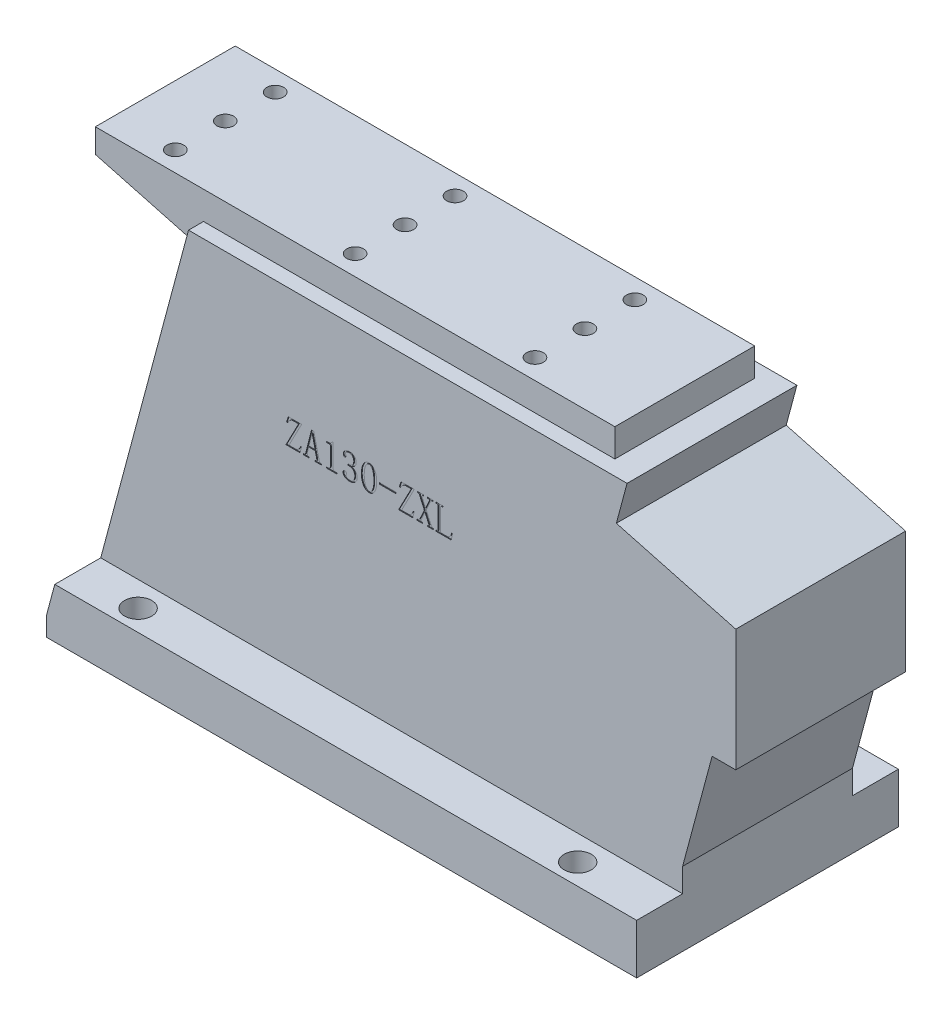
from build123d import *

# Parameters (mm, degrees)
BOSS_EXTRUDE1_DEPTH   = 21.25
SKETCH2_W             = 130
SKETCH2_H             = 3.75
CUT_EXTRUDE1_DEPTH    = 7
CUT_EXTRUDE2_DEPTH    = 3.75
CUT_EXTRUDE3_DEPTH    = 3.75
BOSS_EXTRUDE2_DEPTH   = 32.75
M8_TAPPED_HOLE1_D     = 6.8
M5_TAPPED_HOLE1_D     = 4.2
M5_TAPPED_HOLE1_DEPTH = 12.4
M5_TAPPED_HOLE1_TIP   = 1.2618073
SKETCH10_W            = 4.088356164
SKETCH10_H            = 0.347945206
CUT_EXTRUDE4_DEPTH    = 0.2
SKETCH11_R            = 3
OUTLET_POSITION_DEPTH = 12


with BuildPart() as part:
    # Sketch1 → Boss-Extrude1 (new, symmetric)
    with BuildSketch(Plane.XY):
        Polygon((0, 0), (-130, 0), (-130, -6), (-104.5, -12.832704407), (-127, -96.803847577), (-127, -101.5), (20.7, -101.5), (20.7, -83.052861599), (28.082767015, -55.5), (34, -55.5), (34, -25), (4.124054476, -16.994764524), (6.802143559, -7), (0, -7), align=None)
    extrude(amount=BOSS_EXTRUDE1_DEPTH, both=True)

    # Sketch2 → Cut-Extrude1 (cut)
    with BuildSketch(Plane(origin=(0, 0, 0), x_dir=(1, 0, 0), z_dir=(0, 1, 0))):
        with Locations((-65, 19.375)):
            Rectangle(SKETCH2_W, SKETCH2_H)
        with Locations((-65, -19.375)):
            Rectangle(SKETCH2_W, SKETCH2_H)
    extrude(amount=-CUT_EXTRUDE1_DEPTH, mode=Mode.SUBTRACT)

    # Sketch3 → Cut-Extrude2 (cut)
    with BuildSketch(Plane.XY.offset(21.25)):
        Polygon((-104.5, -12.832704407), (-102.937131564, -7), (-126.267949192, -7), align=None)
    extrude(amount=-CUT_EXTRUDE2_DEPTH, mode=Mode.SUBTRACT)

    # Sketch4 → Cut-Extrude3 (cut)
    with BuildSketch(Plane(origin=(0, 0, -21.25), x_dir=(-1, 0, 0), z_dir=(0, 0, -1))):
        Polygon((102.937131564, -7), (104.5, -12.832704407), (126.267949192, -7), align=None)
    extrude(amount=-CUT_EXTRUDE3_DEPTH, mode=Mode.SUBTRACT)

    # Sketch5 → Boss-Extrude2 (add, symmetric)
    with BuildSketch(Plane.XY):
        Polygon((20.7, -101.5), (20.7, -89), (-124.908965344, -89), (-127, -96.803847577), (-127, -101.5), align=None)
    extrude(amount=BOSS_EXTRUDE2_DEPTH, both=True)

    # M8 Tapped Hole1 (through all)
    with Locations(Plane(origin=(0, -101.5, 0), x_dir=(-1, 0, 0), z_dir=(0, -1, 0))):
        with Locations((-0.7, -27.5), (109.3, -27.5), (-0.7, 27.5), (109.3, 27.5)):
            Hole(M8_TAPPED_HOLE1_D / 2)

    # M5 Tapped Hole1
    with Locations(Plane(origin=(0, 0, 0), x_dir=(1, 0, 0), z_dir=(0, 1, 0))):
        with Locations((-25, 0), (-115, 12.5), (-115, -12.5), (-115, 0), (-70, 12.5), (-70, -12.5), (-70, 0), (-25, 12.5), (-25, -12.5)):
            Hole(M5_TAPPED_HOLE1_D / 2, depth=M5_TAPPED_HOLE1_DEPTH)
            with Locations((0, 0, -(M5_TAPPED_HOLE1_DEPTH + M5_TAPPED_HOLE1_TIP / 2))):  # 118° drill point
                Cone(0, M5_TAPPED_HOLE1_D / 2, M5_TAPPED_HOLE1_TIP, mode=Mode.SUBTRACT)

    # Sketch10 → Cut-Extrude4 (cut)
    # profile 1 of 9: a face of its own
    with BuildSketch(Plane.XY.offset(21.25)):
        with BuildLine():
            add(Edge.make_bspline(
                [(-76.242874665, -41.028711733), (-76.203886828, -41.027431457), (-76.127040008, -41.024907974), (-76.013494906, -41.011969414), (-75.904757802, -40.986452399), (-75.798985146, -40.954804143), (-75.698746914, -40.910149848), (-75.600937291, -40.859034731), (-75.509116676, -40.795612853), (-75.419480888, -40.724507175), (-75.334714639, -40.643281232), (-75.253475154, -40.552312423), (-75.176950666, -40.451930765), (-75.10230024, -40.343014665), (-75.03582371, -40.222632516), (-74.969440865, -40.094612706), (-74.908945483, -39.95631791), (-74.872425189, -39.859995456), (-74.853812165, -39.810903514)],
                knots=[0, 0, 0, 0, 0.944510353, 1.861673376, 2.761280467, 3.64611623, 4.530611868, 5.414086345, 6.314763123, 7.227980775, 8.182441956, 9.153653734, 10.17841272, 11.237309815, 12.347695367, 13.505623519, 14.728709846, 16, 16, 16, 16], degree=3))
            Line((-74.853812165, -39.810903514), (-74.63498725, -39.810903514))
            Line((-74.63498725, -39.810903514), (-75.037298894, -41.289670637))
            Line((-75.037298894, -41.289670637), (-78.549370812, -41.289670637))
            Line((-78.549370812, -41.289670637), (-75.368934168, -35.200629541))
            Line((-75.368934168, -35.200629541), (-76.637031343, -35.200629541))
            add(Edge.make_bspline(
                [(-76.637031343, -35.200629541), (-76.713929015, -35.20386524), (-76.86554004, -35.210244727), (-77.0867771, -35.266142831), (-77.296788501, -35.354772843), (-77.494614616, -35.481230446), (-77.680673118, -35.64201888), (-77.853401182, -35.839278631), (-78.016181535, -36.070275987), (-78.109407187, -36.242043857), (-78.157932456, -36.331451459)],
                knots=[0, 0, 0, 0, 0.92088507, 1.815611915, 2.718761103, 3.64423436, 4.618919569, 5.657996246, 6.78095397, 8, 8, 8, 8], degree=3))
            Line((-78.157932456, -36.331451459), (-78.375398209, -36.244465158))
            Line((-78.375398209, -36.244465158), (-77.939107541, -34.939670637))
            Line((-77.939107541, -34.939670637), (-74.63498725, -34.939670637))
            Line((-74.63498725, -34.939670637), (-77.815423894, -41.028711733))
            Line((-77.815423894, -41.028711733), (-76.242874665, -41.028711733))
        make_face()
    # profile 2 of 9: a face of its own
    with BuildSketch(Plane.XY.offset(21.25)):
        with BuildLine():
            Line((-71.216697439, -38.9410405), (-72.865359682, -38.9410405))
            Line((-72.865359682, -38.9410405), (-73.195635795, -40.298842298))
            add(Edge.make_bspline(
                [(-73.195635795, -40.298842298), (-73.201385906, -40.327331199), (-73.212207931, -40.380948874), (-73.222817521, -40.457693122), (-73.230212975, -40.525684008), (-73.231658112, -40.568393726), (-73.232333141, -40.588343582)],
                knots=[0, 0, 0, 0, 1.193188097, 2.245645547, 3.180534975, 4, 4, 4, 4], degree=3))
            add(Edge.make_bspline(
                [(-73.232333141, -40.588343582), (-73.229172539, -40.637388853), (-73.222745637, -40.737119608), (-73.193404116, -40.860269091), (-73.140700756, -40.950837825), (-73.069099444, -40.998644876), (-72.97445228, -41.024203716), (-72.904047344, -41.027113049), (-72.865359682, -41.028711733)],
                knots=[0, 0, 0, 0, 1.327183477, 2.698751724, 3.381033576, 4.100799874, 4.956385495, 6, 6, 6, 6], degree=3))
            Line((-72.865359682, -41.028711733), (-72.755267644, -41.028711733))
            Line((-72.755267644, -41.028711733), (-72.755267644, -41.289670637))
            Line((-72.755267644, -41.289670637), (-74.113069442, -41.289670637))
            Line((-74.113069442, -41.289670637), (-74.113069442, -41.028711733))
            Line((-74.113069442, -41.028711733), (-74.002977404, -41.028711733))
            add(Edge.make_bspline(
                [(-74.002977404, -41.028711733), (-73.979277578, -41.027869149), (-73.932540679, -41.026207544), (-73.865457949, -41.006905979), (-73.80171868, -40.980398661), (-73.743506339, -40.940084995), (-73.69235851, -40.885762933), (-73.649466648, -40.816358215), (-73.619058841, -40.729997868), (-73.606186651, -40.666913718), (-73.5993066, -40.633195894)],
                knots=[0, 0, 0, 0, 0.909603974, 1.793771294, 2.668600383, 3.558767937, 4.496366253, 5.522416659, 6.675757406, 8, 8, 8, 8], degree=3))
            Line((-73.5993066, -40.633195894), (-72.169469271, -34.939670637))
            Line((-72.169469271, -34.939670637), (-71.620368243, -34.852684336))
            Line((-71.620368243, -34.852684336), (-70.22722826, -40.626400089))
            add(Edge.make_bspline(
                [(-70.22722826, -40.626400089), (-70.214798708, -40.660671284), (-70.191446746, -40.725058124), (-70.147952049, -40.811446769), (-70.100303286, -40.882599979), (-70.047026521, -40.938135249), (-69.987813356, -40.978759842), (-69.924729189, -41.007250277), (-69.857252558, -41.026105198), (-69.810545038, -41.027834713), (-69.78686011, -41.028711733)],
                knots=[0, 0, 0, 0, 1.359311801, 2.55380043, 3.599420041, 4.543802956, 5.406592952, 6.26139706, 7.118371362, 8, 8, 8, 8], degree=3))
            Line((-69.78686011, -41.028711733), (-69.676768072, -41.028711733))
            Line((-69.676768072, -41.028711733), (-69.676768072, -41.289670637))
            Line((-69.676768072, -41.289670637), (-71.254753945, -41.289670637))
            Line((-71.254753945, -41.289670637), (-71.254753945, -41.028711733))
            Line((-71.254753945, -41.028711733), (-71.107964562, -41.028711733))
            add(Edge.make_bspline(
                [(-71.107964562, -41.028711733), (-71.074722312, -41.028173841), (-71.015782969, -41.027220145), (-70.938845974, -41.009815927), (-70.880539429, -40.983149607), (-70.84058845, -40.926410966), (-70.822653035, -40.854167587), (-70.816982114, -40.797688263), (-70.814385795, -40.771830312)],
                knots=[0, 0, 0, 0, 1.306477298, 2.316417055, 3.107965527, 3.758448528, 4.973749602, 6, 6, 6, 6], degree=3))
            add(Edge.make_bspline(
                [(-70.814385795, -40.771830312), (-70.815629301, -40.725782798), (-70.817957288, -40.639576536), (-70.840555758, -40.556409946), (-70.851083141, -40.517667213)],
                knots=[0, 0, 0, 0, 1.068310181, 2, 2, 2, 2], degree=3))
            Line((-70.851083141, -40.517667213), (-71.216697439, -38.9410405))
        make_face()
        Polygon((-71.985982541, -35.563525517), (-72.022679887, -35.563525517), (-72.79196499, -38.680081596), (-71.253394784, -38.680081596), align=None, mode=Mode.SUBTRACT)
    # profile 3 of 9: a face of its own
    with BuildSketch(Plane.XY.offset(21.25)):
        with BuildLine():
            Line((-66.806220127, -34.852684336), (-66.806220127, -40.440195038))
            add(Edge.make_bspline(
                [(-66.806220127, -40.440195038), (-66.80467875, -40.486687653), (-66.801754974, -40.57487759), (-66.765206281, -40.697367598), (-66.707173198, -40.801979197), (-66.624651324, -40.88647853), (-66.521171511, -40.95075514), (-66.399845762, -40.99681991), (-66.260091344, -41.02370043), (-66.161195339, -41.026979912), (-66.108970555, -41.028711733)],
                knots=[0, 0, 0, 0, 1.071056132, 2.031642504, 2.922379843, 3.810776537, 4.728479874, 5.716066906, 6.793905654, 8, 8, 8, 8], degree=3))
            Line((-66.108970555, -41.028711733), (-65.741997096, -41.028711733))
            Line((-65.741997096, -41.028711733), (-65.741997096, -41.289670637))
            Line((-65.741997096, -41.289670637), (-68.442649921, -41.289670637))
            Line((-68.442649921, -41.289670637), (-68.442649921, -41.028711733))
            Line((-68.442649921, -41.028711733), (-68.112373808, -41.028711733))
            add(Edge.make_bspline(
                [(-68.112373808, -41.028711733), (-68.055160572, -41.02707448), (-67.948596144, -41.024024958), (-67.801293568, -40.997405203), (-67.677912998, -40.953587743), (-67.579028914, -40.8883489), (-67.504418159, -40.80282752), (-67.450235877, -40.700325183), (-67.421300953, -40.578541929), (-67.417258166, -40.492439055), (-67.415124236, -40.446990843)],
                knots=[0, 0, 0, 0, 1.316051353, 2.45125549, 3.431393499, 4.310694105, 5.145582167, 6.017928727, 6.953791053, 8, 8, 8, 8], degree=3))
            Line((-67.415124236, -40.446990843), (-67.415124236, -36.050105141))
            add(Edge.make_bspline(
                [(-67.415124236, -36.050105141), (-67.415945488, -36.02686197), (-67.417534132, -35.981899959), (-67.436165212, -35.918269114), (-67.464891325, -35.860912516), (-67.506211557, -35.81159128), (-67.558943345, -35.77127469), (-67.623554665, -35.742634771), (-67.699146587, -35.72483495), (-67.75344712, -35.723337466), (-67.782097695, -35.72254735)],
                knots=[0, 0, 0, 0, 0.998431823, 1.931384586, 2.83044576, 3.74504897, 4.678001734, 5.664921659, 6.767943239, 8, 8, 8, 8], degree=3))
            Line((-67.782097695, -35.72254735), (-68.442649921, -35.72254735))
            Line((-68.442649921, -35.72254735), (-68.442649921, -35.461588445))
            Line((-68.442649921, -35.461588445), (-68.112373808, -35.461588445))
            add(Edge.make_bspline(
                [(-68.112373808, -35.461588445), (-68.042041194, -35.459948587), (-67.907537058, -35.45681252), (-67.7159154, -35.42814996), (-67.544083534, -35.38151405), (-67.391738478, -35.313706281), (-67.256629308, -35.227899375), (-67.139864476, -35.120764029), (-67.037235987, -34.996458), (-66.985047444, -34.901225686), (-66.958446154, -34.852684336)],
                knots=[0, 0, 0, 0, 1.220065567, 2.333254132, 3.353979704, 4.300888212, 5.216996827, 6.11885441, 7.041151654, 8, 8, 8, 8], degree=3))
            Line((-66.958446154, -34.852684336), (-66.806220127, -34.852684336))
        make_face()
    # profile 4 of 9: a face of its own
    with BuildSketch(Plane.XY.offset(21.25)):
        with BuildLine():
            add(Edge.make_bspline(
                [(-60.717179031, -39.525479713), (-60.718632719, -39.583122003), (-60.721496409, -39.696674284), (-60.747683396, -39.863945469), (-60.785780016, -40.026659684), (-60.84458396, -40.183418132), (-60.915732944, -40.336227421), (-61.00571177, -40.482588724), (-61.110480389, -40.624274897), (-61.230837318, -40.759053152), (-61.363979104, -40.8850466), (-61.514099457, -40.992040255), (-61.674525485, -41.085644865), (-61.848763453, -41.159952901), (-62.034728022, -41.219353865), (-62.234102437, -41.258406897), (-62.4457243, -41.28588111), (-62.591366388, -41.28838422), (-62.666215846, -41.289670637)],
                knots=[0, 0, 0, 0, 0.939588951, 1.85094084, 2.756099325, 3.660865542, 4.576551747, 5.501761, 6.458057624, 7.447364816, 8.446121927, 9.440961631, 10.44742643, 11.470200686, 12.524293599, 13.62578974, 14.779828329, 16, 16, 16, 16], degree=3))
            add(Edge.make_bspline(
                [(-62.666215846, -41.289670637), (-62.720648414, -41.28885503), (-62.827548627, -41.287253257), (-62.98445019, -41.267838117), (-63.13641713, -41.2424934), (-63.281610177, -41.200086677), (-63.422710616, -41.150685482), (-63.55715243, -41.087810708), (-63.685575093, -41.013815991), (-63.806948356, -40.930725812), (-63.91740262, -40.838712828), (-64.015600037, -40.743079357), (-64.097976582, -40.643140114), (-64.165254558, -40.540081082), (-64.219681891, -40.434004815), (-64.255334047, -40.322736055), (-64.280519407, -40.209360298), (-64.282583011, -40.13225689), (-64.283617387, -40.093608993)],
                knots=[0, 0, 0, 0, 1.178422216, 2.31430543, 3.421283865, 4.511956533, 5.586120769, 6.657546332, 7.721528688, 8.794167313, 9.839701404, 10.832154961, 11.759582411, 12.638864268, 13.494774353, 14.332771034, 15.164305512, 16, 16, 16, 16], degree=3))
            add(Edge.make_bspline(
                [(-64.283617387, -40.093608993), (-64.281964891, -40.058028558), (-64.278729816, -39.988373108), (-64.247767013, -39.888342875), (-64.202225676, -39.793835003), (-64.134658042, -39.712443263), (-64.062157498, -39.641286677), (-63.984698109, -39.590677598), (-63.908279812, -39.555015851), (-63.855381914, -39.551603863), (-63.829657627, -39.54994461)],
                knots=[0, 0, 0, 0, 1.101766282, 2.156916416, 3.226505383, 4.338286303, 5.423034469, 6.367313602, 7.206023381, 8, 8, 8, 8], degree=3))
            add(Edge.make_bspline(
                [(-63.829657627, -39.54994461), (-63.794496502, -39.551317894), (-63.727550751, -39.553932586), (-63.63588479, -39.585713227), (-63.559963781, -39.638421443), (-63.50763681, -39.711338831), (-63.467382417, -39.786572696), (-63.436808565, -39.857360708), (-63.417296152, -39.921763456), (-63.414876668, -39.96302044), (-63.413754373, -39.982157795)],
                knots=[0, 0, 0, 0, 1.261452964, 2.401769415, 3.443008139, 4.53625006, 5.594855579, 6.516052044, 7.311659842, 8, 8, 8, 8], degree=3))
            add(Edge.make_bspline(
                [(-63.413754373, -39.982157795), (-63.414350208, -40.010768638), (-63.415492744, -40.065631085), (-63.429231137, -40.143365007), (-63.451349155, -40.212949651), (-63.475497074, -40.252550603), (-63.487149065, -40.271659079)],
                knots=[0, 0, 0, 0, 1.131339522, 2.169389213, 3.1166833, 4, 4, 4, 4], degree=3))
            add(Edge.make_bspline(
                [(-63.487149065, -40.271659079), (-63.498740934, -40.294480658), (-63.520738347, -40.337788234), (-63.541137591, -40.404251701), (-63.558510961, -40.46468712), (-63.55989365, -40.504421644), (-63.560543757, -40.523103856)],
                knots=[0, 0, 0, 0, 1.159795864, 2.200897025, 3.154105307, 4, 4, 4, 4], degree=3))
            add(Edge.make_bspline(
                [(-63.560543757, -40.523103856), (-63.557169653, -40.558716386), (-63.550391972, -40.630252528), (-63.49168159, -40.729179466), (-63.402007862, -40.817158468), (-63.279651686, -40.889131327), (-63.139875823, -40.950482171), (-62.988600468, -40.994873139), (-62.830375755, -41.023294596), (-62.722518295, -41.026883515), (-62.667575007, -41.028711733)],
                knots=[0, 0, 0, 0, 0.760241701, 1.527124279, 2.408280577, 3.440242905, 4.55626344, 5.683648738, 6.820035678, 8, 8, 8, 8], degree=3))
            add(Edge.make_bspline(
                [(-62.667575007, -41.028711733), (-62.613593683, -41.027983843), (-62.508439924, -41.026565938), (-62.356220299, -41.006497255), (-62.21366356, -40.977176082), (-62.08154284, -40.935734321), (-61.960934484, -40.880145745), (-61.849155702, -40.815609068), (-61.750107575, -40.735239989), (-61.658766572, -40.645399848), (-61.58000347, -40.541050761), (-61.511792566, -40.42403659), (-61.45275527, -40.29461866), (-61.407512141, -40.150503638), (-61.371219725, -39.99415154), (-61.343476108, -39.824894561), (-61.329488206, -39.642606539), (-61.327241386, -39.516891624), (-61.326083141, -39.452085021)],
                knots=[0, 0, 0, 0, 1.090129821, 2.123535311, 3.096787237, 4.029129623, 4.91414836, 5.776184395, 6.629816794, 7.484381562, 8.359686036, 9.262567746, 10.217298065, 11.227777599, 12.309299728, 13.459264401, 14.690239391, 16, 16, 16, 16], degree=3))
            add(Edge.make_bspline(
                [(-61.326083141, -39.452085021), (-61.326925986, -39.398114666), (-61.328566972, -39.293036519), (-61.347188681, -39.13948513), (-61.375296777, -38.993975317), (-61.414440211, -38.855824286), (-61.466228964, -38.725938903), (-61.530495026, -38.604585456), (-61.605719433, -38.491327374), (-61.691666487, -38.38472628), (-61.7941926, -38.288262438), (-61.917893999, -38.205833494), (-62.061200058, -38.137843067), (-62.223509758, -38.079792681), (-62.406114963, -38.03789006), (-62.608258214, -38.006905032), (-62.830319987, -37.987986361), (-62.985127358, -37.985491464), (-63.065809168, -37.984191185)],
                knots=[0, 0, 0, 0, 0.987551578, 1.922723893, 2.82711971, 3.698668068, 4.547301657, 5.382082243, 6.207914943, 7.033080975, 7.883981262, 8.774232745, 9.742403166, 10.781249731, 11.923906302, 13.166162854, 14.523073474, 16, 16, 16, 16], degree=3))
            Line((-63.065809168, -37.984191185), (-63.065809168, -37.723232281))
            add(Edge.make_bspline(
                [(-63.065809168, -37.723232281), (-63.004609643, -37.722250726), (-62.886057272, -37.720349312), (-62.7147747, -37.70403391), (-62.555689745, -37.676969054), (-62.40906044, -37.639445203), (-62.274195809, -37.590834702), (-62.153070862, -37.529010216), (-62.042943974, -37.458436446), (-61.94597263, -37.376293898), (-61.861065577, -37.284241743), (-61.787290788, -37.183625524), (-61.726025861, -37.073124396), (-61.674035505, -36.955145321), (-61.634492573, -36.827903), (-61.60846684, -36.692431136), (-61.589398225, -36.54899854), (-61.587842362, -36.45022003), (-61.587042045, -36.399409507)],
                knots=[0, 0, 0, 0, 1.294505155, 2.507644584, 3.635876549, 4.705249642, 5.705923862, 6.661804556, 7.576329566, 8.467296251, 9.342240041, 10.220275794, 11.100036209, 12.009979125, 12.943690326, 13.911747118, 14.925826876, 16, 16, 16, 16], degree=3))
            add(Edge.make_bspline(
                [(-61.587042045, -36.399409507), (-61.587712779, -36.357240024), (-61.589036265, -36.274031576), (-61.60292224, -36.151263823), (-61.62643314, -36.03238142), (-61.657415895, -35.917378721), (-61.696447395, -35.805807815), (-61.748008397, -35.699878081), (-61.805675064, -35.596668154), (-61.872543105, -35.498616995), (-61.94701552, -35.406806645), (-62.036003204, -35.328841772), (-62.133995754, -35.261888684), (-62.242384353, -35.207373849), (-62.360553932, -35.164794145), (-62.489337297, -35.135872614), (-62.627982297, -35.115748203), (-62.724129192, -35.114358261), (-62.773589562, -35.11364324)],
                knots=[0, 0, 0, 0, 1.022695627, 2.017973926, 2.992275986, 3.960109165, 4.905719367, 5.854581617, 6.814330317, 7.771558333, 8.731307033, 9.673269304, 10.63049732, 11.603744907, 12.608505999, 13.669579734, 14.801173487, 16, 16, 16, 16], degree=3))
            add(Edge.make_bspline(
                [(-62.773589562, -35.11364324), (-62.818982041, -35.115387796), (-62.911676246, -35.118950285), (-63.052921964, -35.143226633), (-63.198412574, -35.183118177), (-63.320154596, -35.227950547), (-63.414548494, -35.271902485), (-63.476729404, -35.310977022), (-63.530456758, -35.354891119), (-63.572019746, -35.406148191), (-63.607271079, -35.460166688), (-63.630148, -35.520944469), (-63.646032845, -35.585803922), (-63.64702491, -35.631381639), (-63.647530058, -35.654589302)],
                knots=[0, 0, 0, 0, 1.436970883, 2.934381968, 4.524552068, 6.208419931, 7.036027663, 7.816025331, 8.528616145, 9.220997879, 9.897598901, 10.560840095, 11.267195891, 12, 12, 12, 12], degree=3))
            add(Edge.make_bspline(
                [(-63.647530058, -35.654589302), (-63.647447232, -35.698252189), (-63.647298184, -35.776824672), (-63.63045143, -35.880097051), (-63.614655923, -35.961697414), (-63.586165229, -35.999011513), (-63.574135367, -36.014766956)],
                knots=[0, 0, 0, 0, 1.395480087, 2.511202148, 3.371372496, 4, 4, 4, 4], degree=3))
            add(Edge.make_bspline(
                [(-63.574135367, -36.014766956), (-63.562618424, -36.026977386), (-63.539785295, -36.051185404), (-63.516952879, -36.095836617), (-63.502577213, -36.14434706), (-63.50136219, -36.178212392), (-63.500740675, -36.195535363)],
                knots=[0, 0, 0, 0, 0.999189914, 1.980962611, 2.967211498, 4, 4, 4, 4], degree=3))
            add(Edge.make_bspline(
                [(-63.500740675, -36.195535363), (-63.501326392, -36.224141412), (-63.502449527, -36.278994666), (-63.516295369, -36.356651051), (-63.537775484, -36.425487171), (-63.567401096, -36.485374301), (-63.608473306, -36.535822829), (-63.666620333, -36.568568512), (-63.735821327, -36.589294153), (-63.786443873, -36.591328951), (-63.813347695, -36.592410363)],
                knots=[0, 0, 0, 0, 1.184719969, 2.271748375, 3.257852842, 4.165131486, 5.031021611, 5.90724081, 6.88778365, 8, 8, 8, 8], degree=3))
            add(Edge.make_bspline(
                [(-63.813347695, -36.592410363), (-63.836600118, -36.59111083), (-63.883104963, -36.588511763), (-63.951091027, -36.566954342), (-64.015753674, -36.531557938), (-64.079290193, -36.485004362), (-64.134694108, -36.417251182), (-64.171929343, -36.32542322), (-64.192087449, -36.212274119), (-64.195037342, -36.129930983), (-64.196631086, -36.085443326)],
                knots=[0, 0, 0, 0, 0.776613644, 1.553227288, 2.360011848, 3.235995281, 4.173283968, 5.245872554, 6.512023158, 8, 8, 8, 8], degree=3))
            add(Edge.make_bspline(
                [(-64.196631086, -36.085443326), (-64.194876606, -36.04096629), (-64.191435857, -35.953741406), (-64.16989056, -35.826011121), (-64.131147803, -35.705099301), (-64.077296715, -35.590614589), (-64.011326412, -35.48056064), (-63.926350005, -35.379725979), (-63.828012108, -35.284070124), (-63.715748505, -35.195914668), (-63.594927061, -35.114504435), (-63.466220908, -35.045789191), (-63.334413975, -34.985516164), (-63.197863255, -34.935771159), (-63.055967511, -34.900063073), (-62.910368886, -34.872419451), (-62.759933785, -34.85570568), (-62.658102648, -34.85370161), (-62.606412764, -34.852684336)],
                knots=[0, 0, 0, 0, 0.956362997, 1.875544358, 2.775058185, 3.677152513, 4.590950628, 5.525080673, 6.503219877, 7.536133433, 8.589736869, 9.631431218, 10.668927377, 11.704180595, 12.750781765, 13.811072819, 14.888892, 16, 16, 16, 16], degree=3))
            add(Edge.make_bspline(
                [(-62.606412764, -34.852684336), (-62.546088604, -34.853827157), (-62.428196984, -34.856060575), (-62.256143399, -34.878236117), (-62.093695134, -34.914836247), (-61.94048421, -34.965717347), (-61.795249661, -35.028445765), (-61.6616293, -35.110559113), (-61.53578342, -35.204018629), (-61.421598722, -35.31163155), (-61.317666645, -35.425521169), (-61.228388673, -35.544158214), (-61.150874521, -35.662996659), (-61.087921216, -35.784525244), (-61.039243563, -35.90807904), (-61.002806898, -36.032985399), (-60.982177678, -36.159956068), (-60.979484187, -36.245301322), (-60.978137935, -36.287958308)],
                knots=[0, 0, 0, 0, 1.203211274, 2.351438074, 3.454578809, 4.520914548, 5.569162387, 6.603281193, 7.64291744, 8.691983599, 9.728825385, 10.716042705, 11.651398645, 12.557101078, 13.441805741, 14.297394086, 15.149009051, 16, 16, 16, 16], degree=3))
            add(Edge.make_bspline(
                [(-60.978137935, -36.287958308), (-60.978765281, -36.333302589), (-60.979997866, -36.422393228), (-60.994317241, -36.553142974), (-61.015810523, -36.678513177), (-61.045685358, -36.799090255), (-61.084916062, -36.914730936), (-61.13421503, -37.024945993), (-61.191426927, -37.129961074), (-61.25684592, -37.229910831), (-61.331720364, -37.323798919), (-61.416377631, -37.411752053), (-61.512393811, -37.490990844), (-61.61605143, -37.567447175), (-61.731612033, -37.634094345), (-61.856479368, -37.695749982), (-61.990707145, -37.751715834), (-62.085163543, -37.782339427), (-62.13342475, -37.797986134)],
                knots=[0, 0, 0, 0, 1.055798875, 2.074391647, 3.059863201, 4.01712999, 4.964926181, 5.900362499, 6.825984601, 7.747990037, 8.679190214, 9.619554446, 10.585680447, 11.57571844, 12.616430663, 13.687779541, 14.818602511, 16, 16, 16, 16], degree=3))
            add(Edge.make_bspline(
                [(-62.13342475, -37.797986134), (-62.0674541, -37.822650306), (-61.939557746, -37.870466384), (-61.758291742, -37.951516706), (-61.594475258, -38.04069111), (-61.445810205, -38.133839569), (-61.31343596, -38.233312883), (-61.196499504, -38.337623761), (-61.098130529, -38.450246087), (-60.989642089, -38.604137781), (-60.883740376, -38.802165643), (-60.787163939, -39.041808823), (-60.728889695, -39.283498621), (-60.721052191, -39.445447398), (-60.717179031, -39.525479713)],
                knots=[0, 0, 0, 0, 1.057801082, 2.050743778, 2.979484943, 3.857393563, 4.683556733, 5.464061344, 6.206680192, 6.924210677, 8.288531046, 9.568685263, 10.798485854, 12, 12, 12, 12], degree=3))
        make_face()
    # profile 5 of 9: a face of its own
    with BuildSketch(Plane.XY.offset(21.25)):
        with BuildLine():
            add(Edge.make_bspline(
                [(-57.740616531, -41.289670637), (-57.80741428, -41.28701094), (-57.939917761, -41.281735027), (-58.133879923, -41.240961674), (-58.320592599, -41.175449226), (-58.49715134, -41.080290666), (-58.666503669, -40.96030664), (-58.826980462, -40.81414421), (-58.978254018, -40.640419541), (-59.121981322, -40.442951327), (-59.252256142, -40.220110595), (-59.364482729, -39.973790169), (-59.461658292, -39.706868559), (-59.537710022, -39.417183078), (-59.599255667, -39.106771891), (-59.641276135, -38.774317316), (-59.669812791, -38.420527729), (-59.672144394, -38.177252779), (-59.673343415, -38.052149233)],
                knots=[0, 0, 0, 0, 0.767250741, 1.521958388, 2.268065715, 3.034467767, 3.819000744, 4.648475774, 5.522893313, 6.462413781, 7.451976165, 8.484150117, 9.569693735, 10.71285997, 11.923041375, 13.204516973, 14.562429716, 16, 16, 16, 16], degree=3))
            add(Edge.make_bspline(
                [(-59.673343415, -38.052149233), (-59.671970476, -37.935663175), (-59.669285133, -37.707827012), (-59.642721321, -37.37479274), (-59.600921244, -37.058497755), (-59.543603301, -36.75936626), (-59.46684135, -36.477978847), (-59.374921402, -36.213764788), (-59.265989086, -35.966163432), (-59.140665152, -35.737691177), (-59.00148142, -35.531472057), (-58.851778015, -35.35056054), (-58.691988669, -35.196299516), (-58.521371086, -35.070103602), (-58.340306737, -34.971861091), (-58.148875662, -34.90436854), (-57.948364335, -34.859602927), (-57.810632468, -34.855016065), (-57.740616531, -34.852684336)],
                knots=[0, 0, 0, 0, 1.350929405, 2.64229538, 3.872315005, 5.050313999, 6.172152271, 7.252456196, 8.292395744, 9.30609947, 10.270994142, 11.173954753, 12.025102958, 12.840728079, 13.62838015, 14.404660392, 15.189009777, 16, 16, 16, 16], degree=3))
            add(Edge.make_bspline(
                [(-57.740616531, -34.852684336), (-57.673830875, -34.855358957), (-57.541795428, -34.860646692), (-57.34835007, -34.900945362), (-57.164305755, -34.968648356), (-56.989074583, -35.06180821), (-56.822975544, -35.18188372), (-56.666107586, -35.328937656), (-56.518122058, -35.502509043), (-56.380086824, -35.7011378), (-56.253974368, -35.922357637), (-56.143359639, -36.165552804), (-56.051957396, -36.430299724), (-55.975601596, -36.71498458), (-55.918023788, -37.020421424), (-55.876483318, -37.3458227), (-55.849886957, -37.691982645), (-55.847285135, -37.929774132), (-55.845946154, -38.052149233)],
                knots=[0, 0, 0, 0, 0.778153865, 1.538412574, 2.291945889, 3.057433073, 3.844514834, 4.674108351, 5.558006296, 6.498621856, 7.489745676, 8.522585327, 9.608286522, 10.751026339, 11.955650623, 13.228468747, 14.573681417, 16, 16, 16, 16], degree=3))
            add(Edge.make_bspline(
                [(-55.845946154, -38.052149233), (-55.847287749, -38.174524986), (-55.849899604, -38.412769615), (-55.876606965, -38.760266384), (-55.917855097, -39.087523328), (-55.975835602, -39.395127935), (-56.051842245, -39.682170938), (-56.144010112, -39.950185866), (-56.253547227, -40.197903722), (-56.380217605, -40.423340119), (-56.517609925, -40.626086943), (-56.666608338, -40.802328217), (-56.822399834, -40.953668182), (-56.989106543, -41.076066927), (-57.16355306, -41.172945065), (-57.34862072, -41.239451992), (-57.541586072, -41.282197019), (-57.673791749, -41.287161358), (-57.740616531, -41.289670637)],
                knots=[0, 0, 0, 0, 1.415839737, 2.756397436, 4.030263173, 5.231186309, 6.375661746, 7.463286936, 8.507661579, 9.505194878, 10.4518357, 11.337222645, 12.171514211, 12.958980414, 13.723818933, 14.471816206, 15.227563059, 16, 16, 16, 16], degree=3))
        make_face()
        with BuildLine():
            add(Edge.make_bspline(
                [(-57.740616531, -35.11364324), (-57.783970096, -35.115787798), (-57.870145495, -35.120050612), (-57.995388121, -35.161323821), (-58.114907673, -35.22461152), (-58.229063875, -35.313584359), (-58.336281638, -35.428099677), (-58.438355965, -35.567299044), (-58.535848814, -35.73057457), (-58.62572905, -35.917887101), (-58.70803321, -36.125521884), (-58.78148015, -36.350918167), (-58.842395323, -36.593464462), (-58.890428422, -36.852863468), (-58.929902058, -37.128511707), (-58.958394166, -37.421445955), (-58.974420811, -37.731204014), (-58.976425554, -37.943397847), (-58.977453004, -38.052149233)],
                knots=[0, 0, 0, 0, 0.602926481, 1.198458081, 1.820257552, 2.482474919, 3.206465472, 4.001317188, 4.885518666, 5.854776195, 6.895475903, 7.998413689, 9.15845504, 10.380291587, 11.675929166, 13.040829135, 14.483396381, 16, 16, 16, 16], degree=3))
            add(Edge.make_bspline(
                [(-58.977453004, -38.052149233), (-58.976443465, -38.166790143), (-58.974483153, -38.389398572), (-58.958388101, -38.713637199), (-58.930132107, -39.017920383), (-58.89059912, -39.302180227), (-58.842656842, -39.567040489), (-58.781826403, -39.812360996), (-58.708497636, -40.037856067), (-58.626028935, -40.243236792), (-58.535850429, -40.426829411), (-58.438450528, -40.586132501), (-58.335921035, -40.721389614), (-58.228645226, -40.833000026), (-58.114873127, -40.920550275), (-57.995296151, -40.982558849), (-57.869922534, -41.021970899), (-57.783939874, -41.02645325), (-57.740616531, -41.028711733)],
                knots=[0, 0, 0, 0, 1.579122384, 3.066322063, 4.470393475, 5.78721928, 7.018605682, 8.176524123, 9.26593442, 10.282286386, 11.222849205, 12.080205747, 12.850358176, 13.556480444, 14.20678368, 14.818064618, 15.404468389, 16, 16, 16, 16], degree=3))
            add(Edge.make_bspline(
                [(-57.740616531, -41.028711733), (-57.695047361, -41.026436432), (-57.604654184, -41.021923036), (-57.473279904, -40.983107332), (-57.349455953, -40.921668308), (-57.235068634, -40.833243754), (-57.12914846, -40.721564554), (-57.02897517, -40.586918394), (-56.938748192, -40.426597006), (-56.856761619, -40.242854996), (-56.782373355, -40.037532592), (-56.717394471, -39.811888408), (-56.663773743, -39.566559841), (-56.619137576, -39.302110921), (-56.58374058, -39.017813652), (-56.560288381, -38.713472763), (-56.544972281, -38.389377526), (-56.542902556, -38.166790422), (-56.541836565, -38.052149233)],
                knots=[0, 0, 0, 0, 0.62681337, 1.243376882, 1.871556672, 2.522077735, 3.224091877, 3.986978459, 4.828682658, 5.753517391, 6.756780902, 7.835557076, 8.986691132, 10.215210923, 11.530034633, 12.932952135, 14.420348669, 16, 16, 16, 16], degree=3))
            add(Edge.make_bspline(
                [(-56.541836565, -38.052149233), (-56.542315188, -37.943394122), (-56.543248996, -37.731209562), (-56.559299293, -37.42167295), (-56.581529374, -37.128739848), (-56.613904175, -36.853003938), (-56.655813982, -36.593989653), (-56.707252059, -36.351693822), (-56.767776892, -36.125913733), (-56.838337279, -35.918533345), (-56.915195943, -35.730265681), (-57.00485251, -35.566758526), (-57.10291419, -35.427207471), (-57.210506393, -35.312410825), (-57.329254498, -35.223486817), (-57.457703371, -35.160080619), (-57.595968782, -35.119922357), (-57.691866126, -35.115759481), (-57.740616531, -35.11364324)],
                knots=[0, 0, 0, 0, 1.50959593, 2.945267988, 4.301729239, 5.587388111, 6.798192857, 7.942949458, 9.024687178, 10.041038677, 10.982531678, 11.843893582, 12.624018766, 13.344707795, 14.018945998, 14.671509177, 15.324647983, 16, 16, 16, 16], degree=3))
        make_face(mode=Mode.SUBTRACT)
    # profile 6 of 9: a face of its own
    with BuildSketch(Plane.XY.offset(21.25)):
        with Locations((-53.105877661, -37.984191185)):
            Rectangle(SKETCH10_W, SKETCH10_H)
    # profile 7 of 9: a face of its own
    with BuildSketch(Plane.XY.offset(21.25)):
        with BuildLine():
            add(Edge.make_bspline(
                [(-48.059313021, -41.028711733), (-48.020325184, -41.027431457), (-47.943478364, -41.024907974), (-47.829933262, -41.011969414), (-47.721196159, -40.986452399), (-47.615423502, -40.954804143), (-47.51518527, -40.910149848), (-47.417375647, -40.859034731), (-47.325555032, -40.795612853), (-47.235919244, -40.724507175), (-47.151152995, -40.643281232), (-47.06991351, -40.552312423), (-46.993389023, -40.451930765), (-46.918738596, -40.343014665), (-46.852262066, -40.222632516), (-46.785879222, -40.094612706), (-46.725383839, -39.95631791), (-46.688863545, -39.859995456), (-46.670250521, -39.810903514)],
                knots=[0, 0, 0, 0, 0.944510353, 1.861673376, 2.761280467, 3.64611623, 4.530611868, 5.414086345, 6.314763123, 7.227980775, 8.182441956, 9.153653734, 10.17841272, 11.237309815, 12.347695367, 13.505623519, 14.728709846, 16, 16, 16, 16], degree=3))
            Line((-46.670250521, -39.810903514), (-46.451425606, -39.810903514))
            Line((-46.451425606, -39.810903514), (-46.85373725, -41.289670637))
            Line((-46.85373725, -41.289670637), (-50.365809168, -41.289670637))
            Line((-50.365809168, -41.289670637), (-47.185372524, -35.200629541))
            Line((-47.185372524, -35.200629541), (-48.453469699, -35.200629541))
            add(Edge.make_bspline(
                [(-48.453469699, -35.200629541), (-48.530367371, -35.20386524), (-48.681978396, -35.210244727), (-48.903215456, -35.266142831), (-49.113226857, -35.354772843), (-49.311052972, -35.481230446), (-49.497111474, -35.64201888), (-49.669839538, -35.839278631), (-49.832619891, -36.070275987), (-49.925845543, -36.242043857), (-49.974370812, -36.331451459)],
                knots=[0, 0, 0, 0, 0.92088507, 1.815611915, 2.718761103, 3.64423436, 4.618919569, 5.657996246, 6.78095397, 8, 8, 8, 8], degree=3))
            Line((-49.974370812, -36.331451459), (-50.191836565, -36.244465158))
            Line((-50.191836565, -36.244465158), (-49.755545897, -34.939670637))
            Line((-49.755545897, -34.939670637), (-46.451425606, -34.939670637))
            Line((-46.451425606, -34.939670637), (-49.63186225, -41.028711733))
            Line((-49.63186225, -41.028711733), (-48.059313021, -41.028711733))
        make_face()
    # profile 8 of 9: a face of its own
    with BuildSketch(Plane.XY.offset(21.25)):
        with BuildLine():
            Line((-43.468067302, -37.899923206), (-42.197251805, -40.625040928))
            add(Edge.make_bspline(
                [(-42.197251805, -40.625040928), (-42.179292526, -40.659372509), (-42.145424352, -40.724116086), (-42.08789566, -40.810868469), (-42.028564998, -40.882497821), (-41.965380236, -40.93839925), (-41.898672338, -40.97789634), (-41.831222066, -41.0071504), (-41.761072592, -41.025988745), (-41.713053277, -41.027801101), (-41.688925606, -41.028711733)],
                knots=[0, 0, 0, 0, 1.352881584, 2.551306755, 3.629456145, 4.594301707, 5.481928241, 6.325713605, 7.158742058, 8, 8, 8, 8], degree=3))
            Line((-41.688925606, -41.028711733), (-41.58019273, -41.028711733))
            Line((-41.58019273, -41.028711733), (-41.58019273, -41.289670637))
            Line((-41.58019273, -41.289670637), (-43.151382798, -41.289670637))
            Line((-43.151382798, -41.289670637), (-43.151382798, -41.028711733))
            Line((-43.151382798, -41.028711733), (-43.004593415, -41.028711733))
            add(Edge.make_bspline(
                [(-43.004593415, -41.028711733), (-42.976924729, -41.027827494), (-42.92772842, -41.026255271), (-42.862451761, -41.018141822), (-42.814317694, -41.002152287), (-42.774802975, -40.969106525), (-42.753712282, -40.913330833), (-42.749753681, -40.868399022), (-42.747711993, -40.845225004)],
                knots=[0, 0, 0, 0, 1.351927217, 2.403794299, 3.209556397, 3.790599709, 4.860480314, 6, 6, 6, 6], degree=3))
            add(Edge.make_bspline(
                [(-42.747711993, -40.845225004), (-42.749571914, -40.820436657), (-42.753398768, -40.769433756), (-42.77388156, -40.722538778), (-42.784409339, -40.69843562)],
                knots=[0, 0, 0, 0, 0.972036741, 2, 2, 2, 2], degree=3))
            Line((-42.784409339, -40.69843562), (-43.758927747, -38.538728856))
            Line((-43.758927747, -38.538728856), (-44.593452576, -40.296123976))
            add(Edge.make_bspline(
                [(-44.593452576, -40.296123976), (-44.604750948, -40.325129263), (-44.626096123, -40.379926796), (-44.656758828, -40.457405774), (-44.680745991, -40.526624121), (-44.695408142, -40.569762718), (-44.702185452, -40.589702743)],
                knots=[0, 0, 0, 0, 1.192989617, 2.253826617, 3.192863389, 4, 4, 4, 4], degree=3))
            add(Edge.make_bspline(
                [(-44.702185452, -40.589702743), (-44.713667261, -40.61119773), (-44.734168057, -40.649577078), (-44.753458058, -40.703167473), (-44.772100083, -40.740779593), (-44.774603683, -40.763117872), (-44.775580144, -40.771830312)],
                knots=[0, 0, 0, 0, 1.479016342, 2.640787105, 3.469875848, 4, 4, 4, 4], degree=3))
            add(Edge.make_bspline(
                [(-44.775580144, -40.771830312), (-44.774887206, -40.794640687), (-44.77360008, -40.837010799), (-44.755323326, -40.894851226), (-44.726335287, -40.941936759), (-44.669961294, -40.989183823), (-44.573793537, -41.02221459), (-44.492192203, -41.026429988), (-44.448022353, -41.028711733)],
                knots=[0, 0, 0, 0, 0.858099361, 1.593913492, 2.263070415, 2.918082398, 4.331793981, 6, 6, 6, 6], degree=3))
            Line((-44.448022353, -41.028711733), (-44.375986822, -41.028711733))
            Line((-44.375986822, -41.028711733), (-44.375986822, -41.289670637))
            Line((-44.375986822, -41.289670637), (-45.755535195, -41.289670637))
            Line((-45.755535195, -41.289670637), (-45.755535195, -41.028711733))
            Line((-45.755535195, -41.028711733), (-45.610104973, -41.028711733))
            add(Edge.make_bspline(
                [(-45.610104973, -41.028711733), (-45.580546161, -41.02741683), (-45.522064815, -41.024854898), (-45.436293017, -41.003921067), (-45.35597493, -40.967944403), (-45.281283433, -40.920208329), (-45.214194139, -40.863046391), (-45.154148492, -40.801280573), (-45.104496718, -40.733643354), (-45.078163951, -40.685604644), (-45.065081428, -40.661738274)],
                knots=[0, 0, 0, 0, 1.025760662, 2.029441008, 3.043916565, 4.069677227, 5.097125989, 6.098707487, 7.055408646, 8, 8, 8, 8], degree=3))
            Line((-45.065081428, -40.661738274), (-43.904357969, -38.207093582))
            Line((-43.904357969, -38.207093582), (-45.13847612, -35.457510963))
            add(Edge.make_bspline(
                [(-45.13847612, -35.457510963), (-45.153614748, -35.42264813), (-45.184324453, -35.351926572), (-45.255408731, -35.283539278), (-45.321689778, -35.238880321), (-45.38118413, -35.216324523), (-45.447253221, -35.20237795), (-45.493592497, -35.201227568), (-45.517682028, -35.200629541)],
                knots=[0, 0, 0, 0, 1.38181518, 2.803103266, 3.535686061, 4.30375599, 5.118205458, 6, 6, 6, 6], degree=3))
            Line((-45.517682028, -35.200629541), (-45.668548894, -35.200629541))
            Line((-45.668548894, -35.200629541), (-45.668548894, -34.939670637))
            Line((-45.668548894, -34.939670637), (-44.147647781, -34.939670637))
            Line((-44.147647781, -34.939670637), (-44.147647781, -35.200629541))
            Line((-44.147647781, -35.200629541), (-44.257739819, -35.200629541))
            add(Edge.make_bspline(
                [(-44.257739819, -35.200629541), (-44.290960992, -35.201552263), (-44.350065336, -35.203193893), (-44.428906112, -35.222857636), (-44.487445642, -35.25748295), (-44.521037851, -35.311746561), (-44.528931462, -35.377149069), (-44.525505541, -35.453604211), (-44.508321567, -35.543515738), (-44.488597796, -35.606767677), (-44.477923894, -35.640997692)],
                knots=[0, 0, 0, 0, 1.253045786, 2.229314647, 3.046299276, 3.754243085, 4.553812188, 5.496303582, 6.645076038, 8, 8, 8, 8], degree=3))
            Line((-44.477923894, -35.640997692), (-43.613497524, -37.590034507))
            Line((-43.613497524, -37.590034507), (-42.755866959, -35.714392384))
            add(Edge.make_bspline(
                [(-42.755866959, -35.714392384), (-42.740197825, -35.674345439), (-42.711555817, -35.601142608), (-42.682048161, -35.496608547), (-42.673426876, -35.407290498), (-42.67896241, -35.331845924), (-42.708220783, -35.268600764), (-42.766345193, -35.227968383), (-42.84322633, -35.203717209), (-42.901514274, -35.20173273), (-42.933917045, -35.200629541)],
                knots=[0, 0, 0, 0, 1.474339253, 2.694982286, 3.708872194, 4.537341015, 5.266696628, 6.009165303, 6.893277818, 8, 8, 8, 8], degree=3))
            Line((-42.933917045, -35.200629541), (-43.148664476, -35.200629541))
            Line((-43.148664476, -35.200629541), (-43.148664476, -34.939670637))
            Line((-43.148664476, -34.939670637), (-41.754165332, -34.939670637))
            Line((-41.754165332, -34.939670637), (-41.754165332, -35.200629541))
            Line((-41.754165332, -35.200629541), (-41.962116959, -35.200629541))
            add(Edge.make_bspline(
                [(-41.962116959, -35.200629541), (-41.974454957, -35.201444716), (-42.001155006, -35.203208796), (-42.042677676, -35.218697948), (-42.088713223, -35.24183291), (-42.158286407, -35.287587261), (-42.249675952, -35.368347711), (-42.309850023, -35.449778354), (-42.342682028, -35.494208308)],
                knots=[0, 0, 0, 0, 0.447941519, 0.969368065, 1.596165285, 2.323363728, 3.993964257, 6, 6, 6, 6], degree=3))
            Line((-42.342682028, -35.494208308), (-43.468067302, -37.899923206))
        make_face()
    # profile 9 of 9: a face of its own
    with BuildSketch(Plane.XY.offset(21.25)):
        with BuildLine():
            add(Edge.make_bspline(
                [(-39.840466702, -40.735132966), (-39.839791969, -40.758419529), (-39.838524732, -40.802154716), (-39.819208569, -40.862874973), (-39.79171846, -40.916153138), (-39.748471959, -40.95717682), (-39.69884075, -40.990037526), (-39.640491494, -41.011249294), (-39.57677088, -41.02748899), (-39.531150099, -41.028293948), (-39.507472267, -41.028711733)],
                knots=[0, 0, 0, 0, 1.104919029, 2.075181364, 3.01292531, 3.929282611, 4.881833956, 5.832424308, 6.874997497, 8, 8, 8, 8], degree=3))
            Line((-39.507472267, -41.028711733), (-38.508488963, -41.028711733))
            add(Edge.make_bspline(
                [(-38.508488963, -41.028711733), (-38.465858868, -41.027602269), (-38.382146173, -41.025423616), (-38.259357257, -41.010212985), (-38.141262689, -40.985349601), (-38.027094224, -40.952118352), (-37.918105369, -40.90676444), (-37.814129881, -40.851871874), (-37.714127001, -40.787819759), (-37.619363384, -40.712822804), (-37.528461021, -40.628120094), (-37.444940753, -40.531510693), (-37.366531568, -40.424364624), (-37.294936728, -40.30579296), (-37.228444071, -40.176276427), (-37.16681425, -40.035851193), (-37.113154775, -39.883773031), (-37.082226474, -39.777984937), (-37.066419185, -39.723917213)],
                knots=[0, 0, 0, 0, 0.968471023, 1.901786038, 2.806215245, 3.708357056, 4.599152206, 5.483201298, 6.376905902, 7.293264722, 8.225386928, 9.195661489, 10.190096855, 11.238728023, 12.339032901, 13.496040909, 14.720239999, 16, 16, 16, 16], degree=3))
            Line((-37.066419185, -39.723917213), (-36.882932456, -39.810903514))
            Line((-36.882932456, -39.810903514), (-37.217286052, -41.289670637))
            Line((-37.217286052, -41.289670637), (-41.036528346, -41.289670637))
            Line((-41.036528346, -41.289670637), (-41.036528346, -41.028711733))
            Line((-41.036528346, -41.028711733), (-40.779646925, -41.028711733))
            add(Edge.make_bspline(
                [(-40.779646925, -41.028711733), (-40.751437828, -41.028376396), (-40.698629389, -41.027748634), (-40.627142043, -41.011950742), (-40.56674449, -40.991889169), (-40.5217888, -40.957291015), (-40.487178318, -40.914617516), (-40.465123973, -40.862275521), (-40.450769638, -40.801595043), (-40.449859204, -40.758337839), (-40.449370812, -40.735132966)],
                knots=[0, 0, 0, 0, 1.319183227, 2.469558204, 3.424729584, 4.274820955, 5.091307053, 5.976025123, 6.91425992, 8, 8, 8, 8], degree=3))
            Line((-40.449370812, -40.735132966), (-40.449370812, -35.494208308))
            add(Edge.make_bspline(
                [(-40.449370812, -35.494208308), (-40.449934789, -35.471026141), (-40.450996881, -35.427369033), (-40.464549527, -35.366392505), (-40.487611815, -35.31449705), (-40.521704825, -35.271919936), (-40.567058822, -35.237819966), (-40.62661093, -35.215190329), (-40.698888044, -35.202282071), (-40.751497203, -35.201205555), (-40.779646925, -35.200629541)],
                knots=[0, 0, 0, 0, 1.085062371, 2.043410581, 2.908232547, 3.724209003, 4.573769755, 5.53611061, 6.681640195, 8, 8, 8, 8], degree=3))
            Line((-40.779646925, -35.200629541), (-40.999831, -35.200629541))
            Line((-40.999831, -35.200629541), (-40.999831, -34.939670637))
            Line((-40.999831, -34.939670637), (-39.253309168, -34.939670637))
            Line((-39.253309168, -34.939670637), (-39.253309168, -35.200629541))
            Line((-39.253309168, -35.200629541), (-39.510190589, -35.200629541))
            add(Edge.make_bspline(
                [(-39.510190589, -35.200629541), (-39.533355903, -35.201285613), (-39.578309844, -35.202558767), (-39.642415089, -35.215901124), (-39.699766432, -35.239835527), (-39.749950079, -35.271547014), (-39.791135798, -35.313563877), (-39.819949349, -35.365632217), (-39.838237178, -35.426864052), (-39.839697067, -35.470960972), (-39.840466702, -35.494208308)],
                knots=[0, 0, 0, 0, 1.107802495, 2.149769703, 3.112213102, 4.068530129, 4.973306959, 5.895838817, 6.890712941, 8, 8, 8, 8], degree=3))
            Line((-39.840466702, -35.494208308), (-39.840466702, -40.735132966))
        make_face()
    extrude(amount=-CUT_EXTRUDE4_DEPTH, mode=Mode.SUBTRACT)

    # Sketch11 → Outlet position (add)
    with BuildSketch(Plane(origin=(0, 0, -21.25), x_dir=(-1, 0, 0), z_dir=(0, 0, -1))):
        with Locations(Location((53.15, -65.5, 0), (0, 0, 180))):
            Circle(SKETCH11_R)
    extrude(amount=OUTLET_POSITION_DEPTH)


solid = part.part
